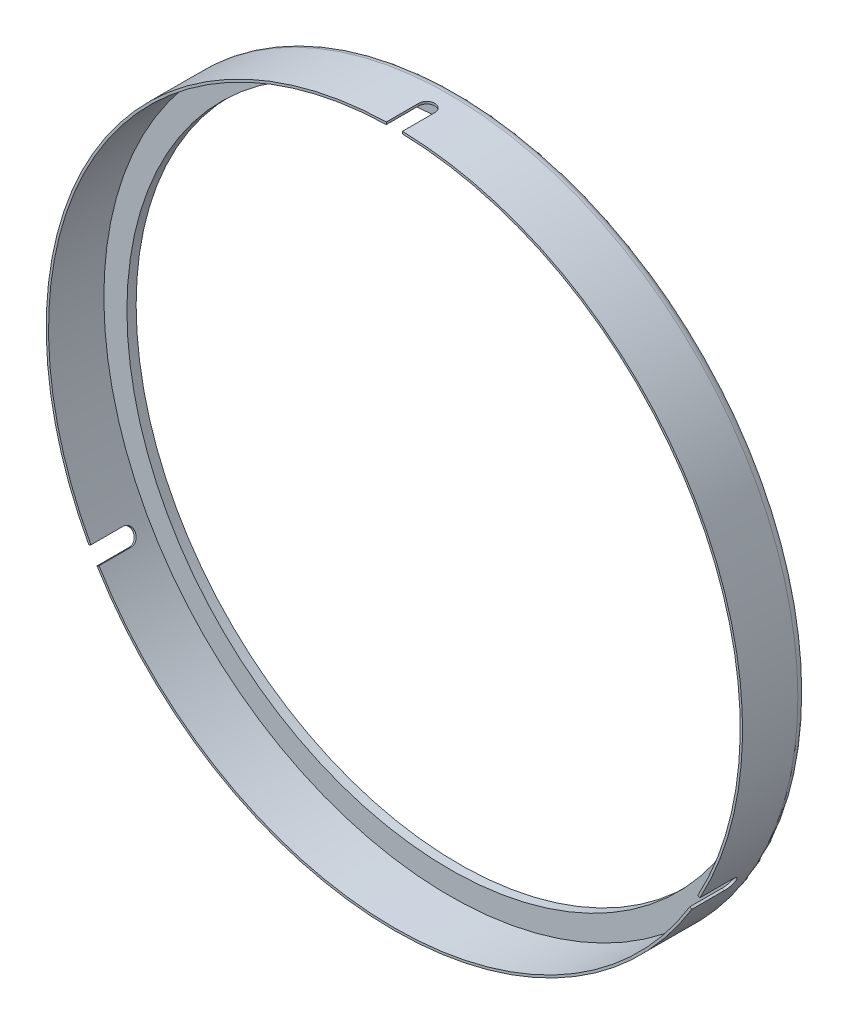
from build123d import *

# Parameters (mm, degrees)
SKETCH_1_R               = 75.5
SKETCH_1_R_2             = 75
BOSS_EXTRUDE_1_DEPTH     = 14
SKETCH_2_R               = 75
BOSS_EXTRUDE_2_DEPTH     = 2
CUT_EXTRUDE_1_REACH      = 109.687
SKETCH_3_R               = 70
CUT_EXTRUDE_3_REACH      = 171.403
CUT_EXTRUDE_3_END_RADIUS = 75
CIRCULAR_PATTERN_1_COUNT = 3
FILLET_1_R               = 2


with BuildPart() as part:
    # Sketch 1 → Boss-Extrude 1 (new body)
    with BuildSketch(Plane.XY):
        Circle(SKETCH_1_R)
        Circle(SKETCH_1_R_2, mode=Mode.SUBTRACT)
    extrude(amount=BOSS_EXTRUDE_1_DEPTH)

    # Sketch 2 → Boss-Extrude 2 (add)
    with BuildSketch(Plane.XY):
        Circle(SKETCH_2_R)
    extrude(amount=BOSS_EXTRUDE_2_DEPTH)

    # Sketch 3 → Cut-Extrude 1 (cut, up to next)
    with BuildSketch(Plane(origin=(0, 0, 0), x_dir=(-1, 0, 0), z_dir=(0, 0, -1)), mode=Mode.PRIVATE) as cut_extrude_1_sk1:
        Circle(SKETCH_3_R)
    cut_extrude_1_tool1 = extrude(cut_extrude_1_sk1.sketch, amount=-CUT_EXTRUDE_1_REACH, mode=Mode.PRIVATE) & part.part
    add(cut_extrude_1_tool1.solids().sort_by_distance((0, 0, 0))[0], mode=Mode.SUBTRACT)

    # Cut-Extrude 3: up to this cylinder (the profile starts outside it)
    cut_extrude_3_end = Plane(origin=(0, 0, 9.803668), z_dir=(0, 0, -1)) * Cylinder(CUT_EXTRUDE_3_END_RADIUS, 493.806, mode=Mode.PRIVATE)
    # Sketch 7 → Cut-Extrude 3 (cut, up to the surface)
    with BuildSketch(Plane(origin=(0, 75.5, 0), x_dir=(1, 0, 0), z_dir=(0, 1, 0)), mode=Mode.PRIVATE) as cut_extrude_3_sk1:
        with BuildLine():
            Line((0, -14), (0, -5.25))
            ThreePointArc((0, -5.25), (-1.237436867, -5.762563133), (-1.75, -7))
            Line((-1.75, -7), (-1.75, -14))
            Line((-1.75, -14), (0, -14))
        make_face()
    cut_extrude_3_tool1 = extrude(cut_extrude_3_sk1.sketch, amount=-CUT_EXTRUDE_3_REACH, mode=Mode.PRIVATE) - cut_extrude_3_end
    # Sketch 7 → Cut-Extrude 3 (cut, up to the surface)
    with BuildSketch(Plane(origin=(0, 75.5, 0), x_dir=(1, 0, 0), z_dir=(0, 1, 0)), mode=Mode.PRIVATE) as cut_extrude_3_sk2:
        with BuildLine():
            ThreePointArc((1.75, -7), (1.237436867, -5.762563133), (0, -5.25))
            Line((0, -5.25), (0, -14))
            Line((0, -14), (1.75, -14))
            Line((1.75, -14), (1.75, -7))
        make_face()
    cut_extrude_3_tool2 = extrude(cut_extrude_3_sk2.sketch, amount=-CUT_EXTRUDE_3_REACH, mode=Mode.PRIVATE) - cut_extrude_3_end
    cut_extrude_3 = cut_extrude_3_tool1.solids().sort_by_distance((-0.85329, 75.5, 9.803668))[0] + cut_extrude_3_tool2.solids().sort_by_distance((0.85329, 75.5, 9.803668))[0]
    add(cut_extrude_3, mode=Mode.SUBTRACT)

    # Circular pattern 1: Cut-Extrude 3 ×3 about axis
    circular_pattern_1_axis = Axis((0, 0, 0), (0, 0, 1))
    for i in range(1, CIRCULAR_PATTERN_1_COUNT):
        add(cut_extrude_3.rotate(circular_pattern_1_axis, i * 360 / CIRCULAR_PATTERN_1_COUNT), mode=Mode.SUBTRACT)

    # Fillet 1
    fillet_1_edges = [part.edges().sort_by_distance(p)[0] for p in [
        (-75.5, 0, 0),
    ]]
    fillet(fillet_1_edges, radius=FILLET_1_R)


solid = part.part
